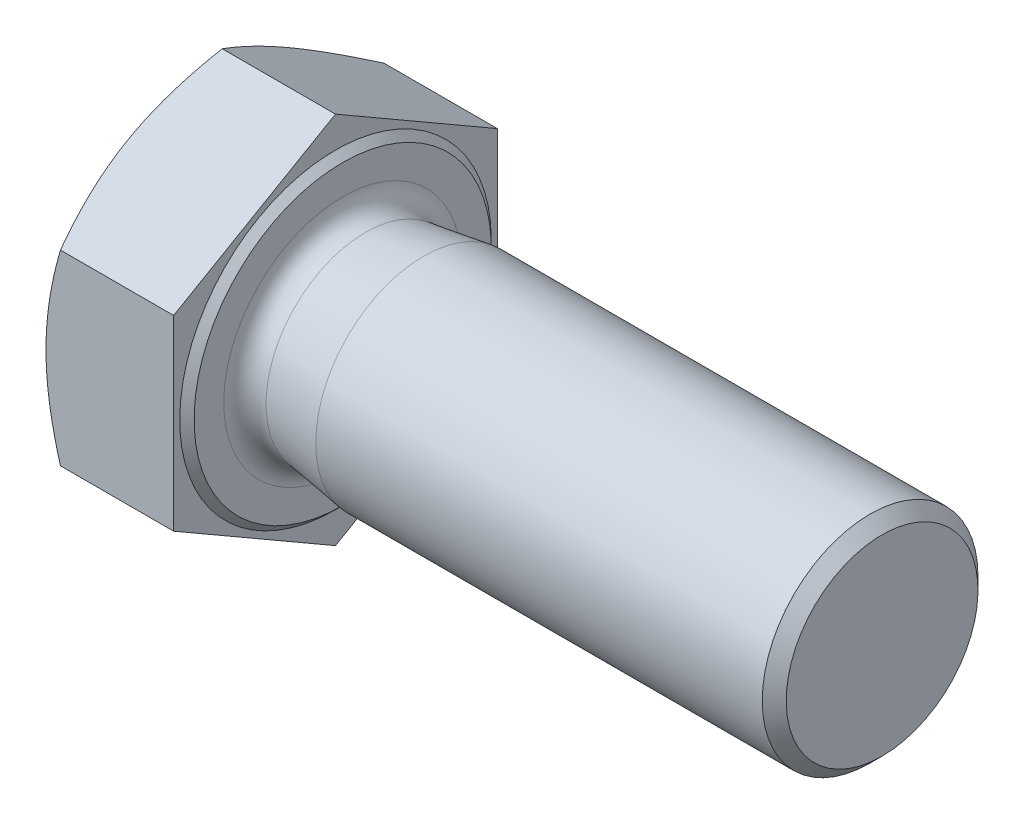
SolidWorks part; units mm, degrees
ref_plane "前视基准面" through (0, 0, 0) normal (0, 0, 1) x (1, 0, 0)
ref_plane "上视基准面" through (0, 0, 0) normal (0, 1, 0) x (1, 0, 0)
ref_plane "右视基准面" through (0, 0, 0) normal (1, 0, 0) x (0, 0, -1)
sketch "草图1" plane through (0, 0, 0) normal (0, 0, 1) x (1, 0, 0)
  line L0 (0, 0) -> (75, 0) construction
  line L1 (0, 0) -> (0, 19.775)
  line L2 (0, 19.775) -> (15, 19.775)
  line L3 (15, 19.775) -> (15, 0)
  line L4 (15, 12) -> (75, 12)
  line L5 (75, 12) -> (75, 0)
  line L6 (0, 18) -> (1.0248, 19.775)
  line L7 (69, 12) -> (69, 0)
  line L8 (24, 12) -> (24, 0)
  line L9 (15, 11.0258) -> (75, 11.0258)
  line L10 (75, 10.3763) -> (15, 10.3763)
  line L11 (14.2, 17.325) -> (15, 16.525)
  line L12 (14.2, 19.775) -> (14.2, 0)
  line L13 (14.9, 16.625) -> (14.9, 0) construction
  arc A0 (15, 14.2) -> (17.2, 12) centre (17.2, 14.2) ccw
  point P12 (72, 0)
  point P13 (5.13, 19.775)
  point P14 (15, 14.2)
  point P24 (15, 16.625)
  dimension "D1" = 0.1
  dimension "r" = 2.2
  dimension "k" = 15
  dimension "D2" = 45
  dimension "β" = 30
  dimension "e" = 39.55
  dimension "s" = 36
  dimension "d" = 24
  dimension "l" = 60
  dimension "D52" = 6
  dimension "P" = 3
  dimension "kw" = 9.87
  dimension "da" = 28.4
  dimension "a" = 9
  dimension "ds" = 22.0515
  dimension "D61" = 20.7525
  dimension "dw" = 33.25
  dimension "c" = 0.8
sketch "草图2" plane through (0, 0, 0) normal (1, 0, 0) x (0, 0, -1)
  line L1 (0, 20.7846) -> (-18, 10.3923)
  line L2 (-18, 10.3923) -> (-18, -10.3923)
  line L3 (-18, -10.3923) -> (0, -20.7846)
  line L4 (0, -20.7846) -> (18, -10.3923)
  line L5 (18, -10.3923) -> (18, 10.3923)
  line L6 (18, 10.3923) -> (0, 20.7846)
  circle A0 centre (0, 0) radius 18 construction
sketch "草图3" plane through (0, 0, 0) normal (1, 0, 0) x (0, 0, -1)
  line L0 (18, 10.3923) -> (0, 20.7846) construction
  line L1 (0, 20.7846) -> (-18, 10.3923) construction
  line L2 (-18, 10.3923) -> (-18, -10.3923) construction
  line L3 (18, -10.3923) -> (18, 10.3923) construction
  line L4 (0, -20.7846) -> (18, -10.3923) construction
  line L5 (-18, -10.3923) -> (0, -20.7846) construction
  line L6 (18, 10.3923) -> (0, 20.7846)
  line L7 (0, 20.7846) -> (-18, 10.3923)
  line L8 (-18, 10.3923) -> (-18, -10.3923)
  line L9 (18, -10.3923) -> (18, 10.3923)
  line L10 (0, -20.7846) -> (18, -10.3923)
  line L11 (-18, -10.3923) -> (0, -20.7846)
extrude "凸台-拉伸1" add sketch "草图3" along normal up to vertex (15 mm away) up to point (15, 19.775, 0)
sketch "草图4" plane through (0, 0, 0) normal (-1, 0, 0) x (0, 0, 1)
  circle A0 centre (0, 0) radius 18 construction
  circle A1 centre (0, 0) radius 18
  circle A2 centre (0, 0) radius 39.55
  dimension "D1" = 79.1
extrude "切除-拉伸1" cut sketch "草图4" against normal blind 1.875 draft 60
sketch "草图5" [suppressed] plane through (0, 0, 0) normal (0, 0, 1) x (1, 0, 0)
  line L0 (35, 28) -> (100, 28) construction
  line L1 (100, 28) -> (100, 0) construction
  line L2 (0, 0) -> (100, 0) construction
  line L3 (40.5, 28) -> (100, 28)
  line L4 (100, 28) -> (100, 0)
  line L5 (35, 0) -> (100, 0)
  line L6 (35, 33.5) -> (35, 0)
  arc A0 (35, 33.5) -> (40.5, 28) centre (40.5, 33.5) ccw construction
  arc A1 (35, 33.5) -> (40.5, 28) centre (40.5, 33.5) ccw
revolve "旋转1" add sketch "草图5" angle 360 about L5
cosmetic thread "装饰螺纹线2" [suppressed] parameters "D1"=51, "D2"=20.7525
chamfer "倒角2" [suppressed] distance 1.3333 angle 45
sketch "草图7" plane through (0, 0, 0) normal (0, 0, 1) x (1, 0, 0)
  line L0 (15, 16.525) -> (14.2, 17.325)
  line L1 (14.2, 17.325) -> (14.2, 39.55)
  line L2 (14.2, 39.55) -> (15, 39.55)
  line L3 (15, 39.55) -> (15, 16.525)
  line L4 (0, 0) -> (75, 0) construction
  line L5 (0, 0) -> (75, 0) construction
  dimension "D1" = 79.1
revolve "切除-旋转1" [suppressed] cut sketch "草图7" angle 360 mid plane about L5
sketch "草图6" plane through (0, 0, 0) normal (0, 0, 1) x (1, 0, 0)
  line L0 (24, 0) -> (24, 12) construction
  line L1 (24, 12) -> (75, 12)
  line L2 (75, 12) -> (75, 0)
  line L3 (24, 12) -> (17.5194, 11.0491)
  line L5 (15, 11.0258) -> (75, 11.0258) construction
  line L6 (15, 19.775) -> (15, 0) construction
  line L7 (15, 13.2257) -> (15, 0)
  line L8 (15, 0) -> (75, 0)
  arc A0 (17.5194, 11.0491) -> (15, 13.2257) centre (17.2, 13.2257) cw
  arc A1 (15, 14.2) -> (17.2, 12) centre (17.2, 14.2) ccw construction
revolve "旋转2" add sketch "草图6" angle 360 about L8
cosmetic thread "装饰螺纹线1" parameters "D1"=51, "D2"=20.7525
chamfer "倒角1" distance 1.3333 angle 45 1 edges at (75, -12, 0)
sketch "草图8" plane through (0, 0, 0) normal (0, 0, 1) x (1, 0, 0)
  line L0 (15, 16.525) -> (14.2, 17.325)
  line L1 (14.2, 17.325) -> (14.2, 39.55)
  line L2 (14.2, 39.55) -> (15, 39.55)
  line L3 (15, 39.55) -> (15, 16.525)
  line L4 (0, 0) -> (75, 0) construction
  line L5 (0, 0) -> (75, 0) construction
  dimension "D1" = 79.1
revolve "切除-旋转2" cut sketch "草图8" angle 360 mid plane about L5
